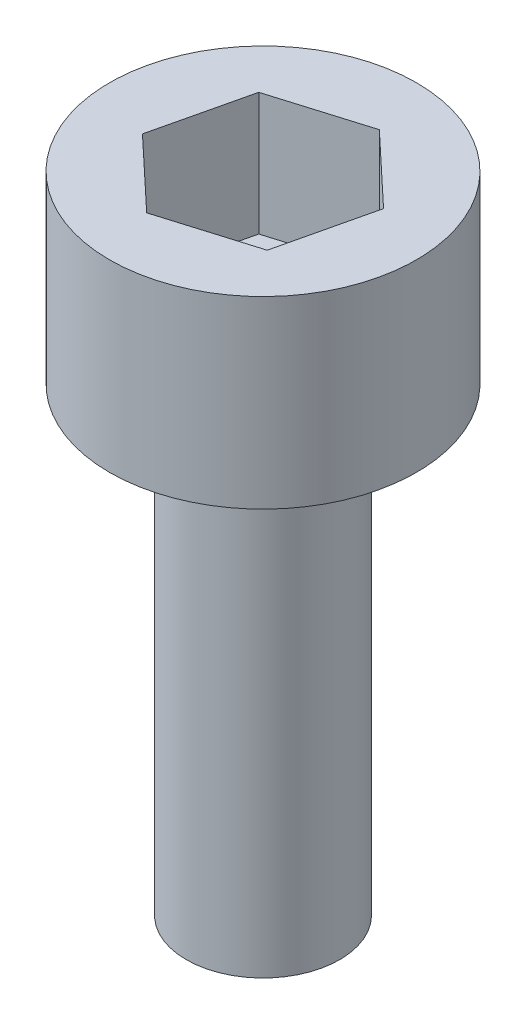
from build123d import *

# Parameters (mm, degrees)
SKETCH1_R           = 5
BOSS_EXTRUDE1_DEPTH = 30
SKETCH2_R           = 10
BOSS_EXTRUDE2_DEPTH = 12
CUT_EXTRUDE1_DEPTH  = 8


with BuildPart() as part:
    # Sketch1 → Boss-Extrude1 (new body)
    with BuildSketch(Plane(origin=(0, 0, 0), x_dir=(1, 0, 0), z_dir=(0, 1, 0))):
        with Locations(Location((0, 0, 0), (0, 0, 270))):
            Circle(SKETCH1_R)
    extrude(amount=BOSS_EXTRUDE1_DEPTH)

    # Sketch2 → Boss-Extrude2 (add)
    with BuildSketch(Plane(origin=(0, 30, 0), x_dir=(1, 0, 0), z_dir=(0, 1, 0))):
        with Locations(Location((0, 0, 0), (0, 0, 270))):
            Circle(SKETCH2_R)
    extrude(amount=BOSS_EXTRUDE2_DEPTH)

    # Sketch3 → Cut-Extrude1 (cut)
    with BuildSketch(Plane(origin=(0, 42, 0), x_dir=(1, 0, 0), z_dir=(0, 1, 0))):
        Polygon((4.59389972, -4.318555573), (6.036928694, 1.819156074), (1.443028974, 6.137711647), (-4.59389972, 4.318555573), (-6.036928694, -1.819156074), (-1.443028974, -6.137711647), align=None)
    extrude(amount=-CUT_EXTRUDE1_DEPTH, mode=Mode.SUBTRACT)


solid = part.part
